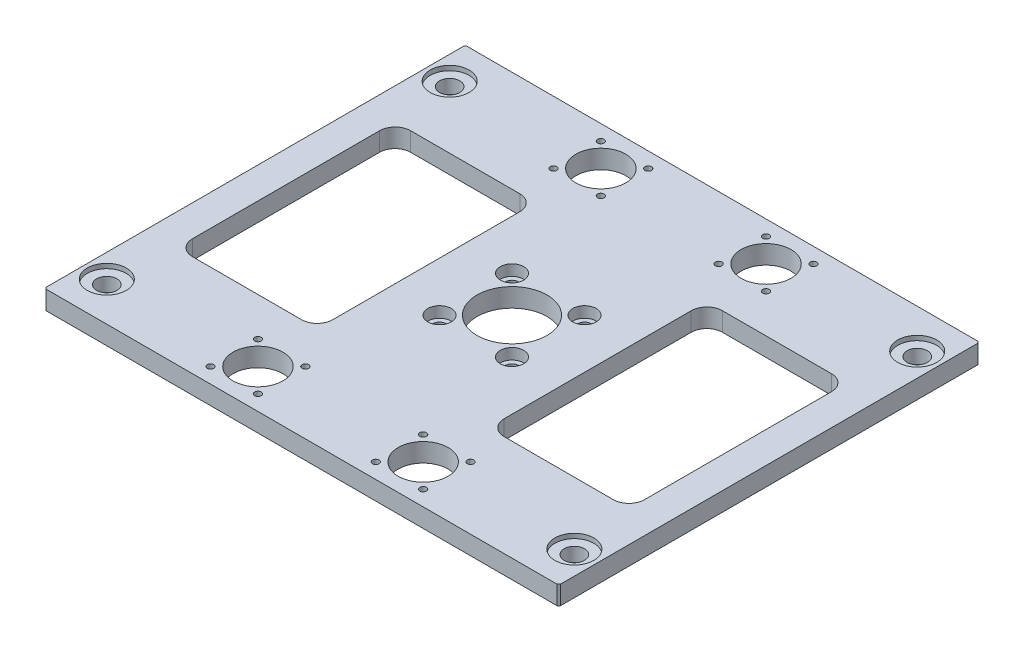
from build123d import *

# Parameters (mm, degrees)
SKETCH1_W                                            = 330
SKETCH1_H                                            = 270
BOSS_EXTRUDE1_DEPTH                                  = 6
SKETCH2_R                                            = 16
CUT_EXTRUDE1_DEPTH                                   = 214.527515791
SKETCH3_R                                            = 22.5
CUT_EXTRUDE2_DEPTH                                   = 214.527515791
SKETCH4_R                                            = 12.5
CUT_EXTRUDE3_DEPTH                                   = 3
M12_CLEARANCE_HOLE1_D                                = 13
M5_TAPPED_HOLE1_D                                    = 4.2
HOLE_SIZE_PER_SOCKET_HEAD_CAP_SCREW_TYPE_D           = 9
HOLE_SIZE_PER_SOCKET_HEAD_CAP_SCREW_TYPE_CBORE_D     = 15
HOLE_SIZE_PER_SOCKET_HEAD_CAP_SCREW_TYPE_CBORE_DEPTH = 7
CHAMFER1_SIZE                                        = 1
CUT_EXTRUDE4_DEPTH                                   = 214.527515791


with BuildPart() as part:
    # Sketch1 → Boss-Extrude1 (new, symmetric)
    with BuildSketch(Plane(origin=(0, 0, 0), x_dir=(1, 0, 0), z_dir=(0, 1, 0))):
        Rectangle(SKETCH1_W, SKETCH1_H)
    extrude(amount=BOSS_EXTRUDE1_DEPTH, both=True)

    # Sketch2 → Cut-Extrude1 (cut, through all)
    with BuildSketch(Plane(origin=(0, 6, 0), x_dir=(1, 0, 0), z_dir=(0, 1, 0))):
        with Locations(Location((-53, 110, 0), (0, 0, 270))):
            Circle(SKETCH2_R)
        with Locations(Location((53, 110, 0), (0, 0, 90))):
            Circle(SKETCH2_R)
        with Locations(Location((53, -110, 0), (0, 0, 270))):
            Circle(SKETCH2_R)
        with Locations(Location((-53, -110, 0), (0, 0, 90))):
            Circle(SKETCH2_R)
    extrude(amount=-CUT_EXTRUDE1_DEPTH, mode=Mode.SUBTRACT)

    # Sketch3 → Cut-Extrude2 (cut, through all)
    with BuildSketch(Plane(origin=(0, 6, 0), x_dir=(1, 0, 0), z_dir=(0, 1, 0))):
        with Locations(Location((0, 0, 0), (0, 0, 270))):
            Circle(SKETCH3_R)
    extrude(amount=-CUT_EXTRUDE2_DEPTH, mode=Mode.SUBTRACT)

    # Sketch4 → Cut-Extrude3 (cut)
    with BuildSketch(Plane(origin=(0, 6, 0), x_dir=(1, 0, 0), z_dir=(0, 1, 0))):
        with Locations(Location((-150, 110, 0), (0, 0, 270))):
            Circle(SKETCH4_R)
        with Locations(Location((150, 110, 0), (0, 0, 90))):
            Circle(SKETCH4_R)
        with Locations(Location((150, -110, 0), (0, 0, 270))):
            Circle(SKETCH4_R)
        with Locations(Location((-150, -110, 0), (0, 0, 90))):
            Circle(SKETCH4_R)
    extrude(amount=-CUT_EXTRUDE3_DEPTH, mode=Mode.SUBTRACT)

    # M12 Clearance Hole1 (through all)
    with Locations(Plane(origin=(0, -6, 0), x_dir=(-1, 0, 0), z_dir=(0, -1, 0))):
        with Locations((150, -110), (-150, -110), (150, 110), (-150, 110)):
            Hole(M12_CLEARANCE_HOLE1_D / 2)

    # M5 Tapped Hole1 (through all)
    with Locations(Plane(origin=(0, 6, 0), x_dir=(1, 0, 0), z_dir=(0, 1, 0))):
        with Locations((-68.202795796, -125.202795796), (-68.202795796, 125.202795796), (-37.797204204, 125.202795796), (-37.797204204, 94.797204204), (-68.202795796, 94.797204204), (37.797204204, 125.202795796), (37.797204204, 94.797204204), (68.202795796, 94.797204204), (68.202795796, 125.202795796), (68.202795796, -125.202795796), (68.202795796, -94.797204204), (37.797204204, -94.797204204), (37.797204204, -125.202795796), (-37.797204204, -125.202795796), (-37.797204204, -94.797204204), (-68.202795796, -94.797204204)):
            Hole(M5_TAPPED_HOLE1_D / 2)

    # Hole size per socket head cap screw type 1 (through all)
    with Locations(Plane(origin=(0, 6, 0), x_dir=(1, 0, 0), z_dir=(0, 1, 0))):
        with Locations((0, 0), (23.25, 23.25), (-23.25, -23.25), (-23.25, 23.25), (23.25, -23.25)):
            CounterBoreHole(HOLE_SIZE_PER_SOCKET_HEAD_CAP_SCREW_TYPE_D / 2, HOLE_SIZE_PER_SOCKET_HEAD_CAP_SCREW_TYPE_CBORE_D / 2, HOLE_SIZE_PER_SOCKET_HEAD_CAP_SCREW_TYPE_CBORE_DEPTH)

    # Chamfer1
    chamfer1_edges = [part.edges().sort_by_distance(p)[0] for p in [
        (165, 0, 135),
        (-165, 0, 135),
        (-165, 0, -135),
        (165, 0, -135),
    ]]
    chamfer(chamfer1_edges, length=CHAMFER1_SIZE)

    # Sketch11 → Cut-Extrude4 (cut, through all)
    with BuildSketch(Plane(origin=(0, 6, 0), x_dir=(1, 0, 0), z_dir=(0, 1, 0))):
        with BuildLine():
            Line((-135, 70), (-65, 70))
            ThreePointArc((-65, 70), (-57.928932188, 67.071067812), (-55, 60))
            Line((-55, 60), (-55, -60))
            ThreePointArc((-55, -60), (-57.928932188, -67.071067812), (-65, -70))
            Line((-65, -70), (-135, -70))
            ThreePointArc((-135, -70), (-142.071067812, -67.071067812), (-145, -60))
            Line((-145, -60), (-145, 60))
            ThreePointArc((-145, 60), (-142.071067812, 67.071067812), (-135, 70))
        make_face()
        with BuildLine():
            Line((55, 60), (55, -60))
            ThreePointArc((55, -60), (57.928932188, -67.071067812), (65, -70))
            Line((65, -70), (135, -70))
            ThreePointArc((135, -70), (142.071067812, -67.071067812), (145, -60))
            Line((145, -60), (145, 60))
            ThreePointArc((145, 60), (142.071067812, 67.071067812), (135, 70))
            Line((135, 70), (65, 70))
            ThreePointArc((65, 70), (57.928932188, 67.071067812), (55, 60))
        make_face()
    extrude(amount=-CUT_EXTRUDE4_DEPTH, mode=Mode.SUBTRACT)


solid = part.part
